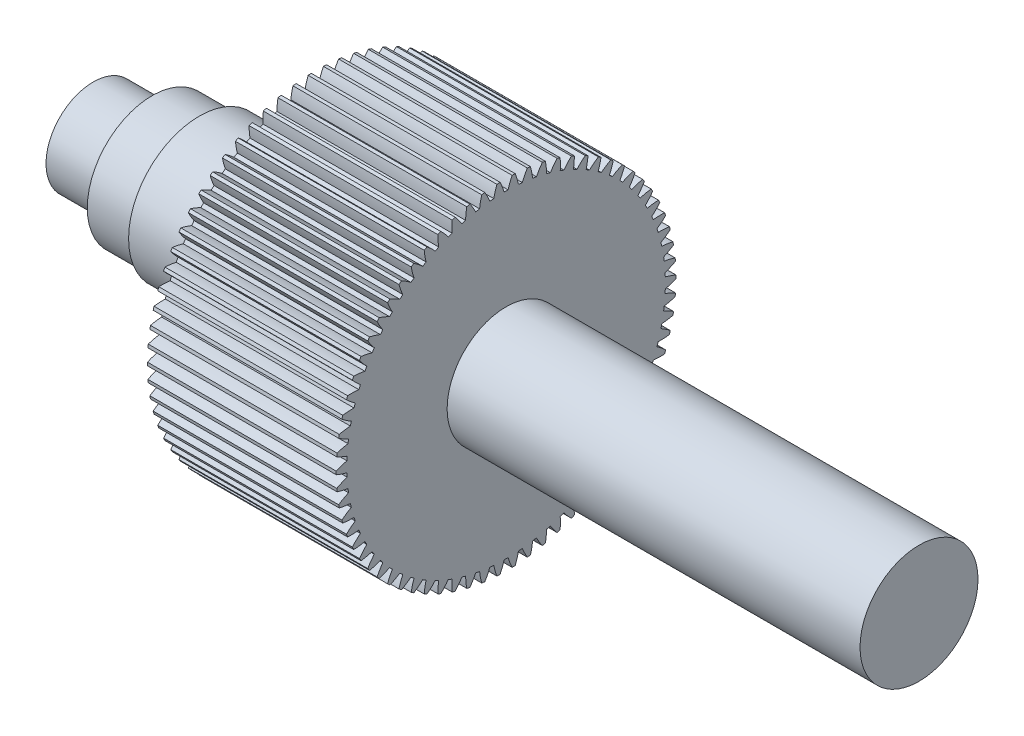
from build123d import *

# Parameters (mm, degrees)
BASPROSKE_W         = 80
BASPROSKE_H         = 72
TOOTHCUT_DEPTH      = 130.49131245
TEETHCUTS_COUNT     = 70
TEETHCUTS_ANGLE     = 354.857142857
BORSKE_R            = 2.5
BORE_DEPTH          = 80.0000508
SKETCH3_R           = 30
BOSS_EXTRUDE3_DEPTH = 50
SKETCH4_R           = 27.5
BOSS_EXTRUDE4_DEPTH = 20
SKETCH5_R           = 20
BOSS_EXTRUDE5_DEPTH = 25
SKETCH6_R           = 25
BOSS_EXTRUDE6_DEPTH = 175


with BuildPart() as part:
    # BasProSke → Base-Revolve (revolve)
    with BuildSketch(Plane(origin=(0, 0, 0), x_dir=(1, 0, 0), z_dir=(0, 1, 0)), mode=Mode.PRIVATE) as base_revolve_sk:
        with Locations((40, 36)):
            Rectangle(BASPROSKE_W, BASPROSKE_H)
    revolve(base_revolve_sk.sketch.rotate(Axis((-10, 0, 0), (1, 0, 0)), 180), axis=Axis((-10, 0, 0), (1, 0, 0)))

    # TooCutSke → ToothCut (cut, through all)
    with BuildSketch(Plane(origin=(0, 0, 0), x_dir=(0, 0, -1), z_dir=(1, 0, 0))):
        with BuildLine():
            ThreePointArc((0.834496205, 67.493841327), (0, 67.499), (-0.834496205, 67.493841327))
            ThreePointArc((-0.834496205, 67.493841327), (-1.607283563, 69.774040651), (-2.573096918, 71.97942357))
            ThreePointArc((-2.573096918, 71.97942357), (0, 72.0254), (2.573096918, 71.97942357))
            ThreePointArc((2.573096918, 71.97942357), (1.607283563, 69.774040651), (0.834496205, 67.493841327))
        make_face()
    toothcut = extrude(amount=TOOTHCUT_DEPTH, mode=Mode.SUBTRACT)

    # TeethCuts: ToothCut ×70 about axis
    teethcuts_axis = Axis((-10, 0, 0), (1, 0, 0))
    for i in range(1, TEETHCUTS_COUNT):
        add(toothcut.rotate(teethcuts_axis, i * TEETHCUTS_ANGLE / (TEETHCUTS_COUNT - 1)), mode=Mode.SUBTRACT)

    # BorSke → Bore (cut, symmetric)
    with BuildSketch(Plane(origin=(0, 0, 0), x_dir=(0, 0, -1), z_dir=(1, 0, 0))):
        with Locations(Location((0, 0, 0), (0, 0, 180))):
            Circle(BORSKE_R)
    extrude(amount=BORE_DEPTH, both=True, mode=Mode.SUBTRACT)

    # Sketch3 → Boss-Extrude3 (add)
    with BuildSketch(Plane.ZY):
        with Locations(Location((0, 0, 0), (0, 0, 180))):
            Circle(SKETCH3_R)
    extrude(amount=BOSS_EXTRUDE3_DEPTH)

    # Sketch4 → Boss-Extrude4 (add)
    with BuildSketch(Plane.ZY.offset(50)):
        Circle(SKETCH4_R)
    extrude(amount=BOSS_EXTRUDE4_DEPTH)

    # Sketch5 → Boss-Extrude5 (add)
    with BuildSketch(Plane.ZY.offset(70)):
        Circle(SKETCH5_R)
    extrude(amount=BOSS_EXTRUDE5_DEPTH)

    # Sketch6 → Boss-Extrude6 (add)
    with BuildSketch(Plane(origin=(80, 0, 0), x_dir=(0, 0, -1), z_dir=(1, 0, 0))):
        with Locations(Location((0, 0, 0), (0, 0, 180))):
            Circle(SKETCH6_R)
    extrude(amount=BOSS_EXTRUDE6_DEPTH)


solid = part.part
